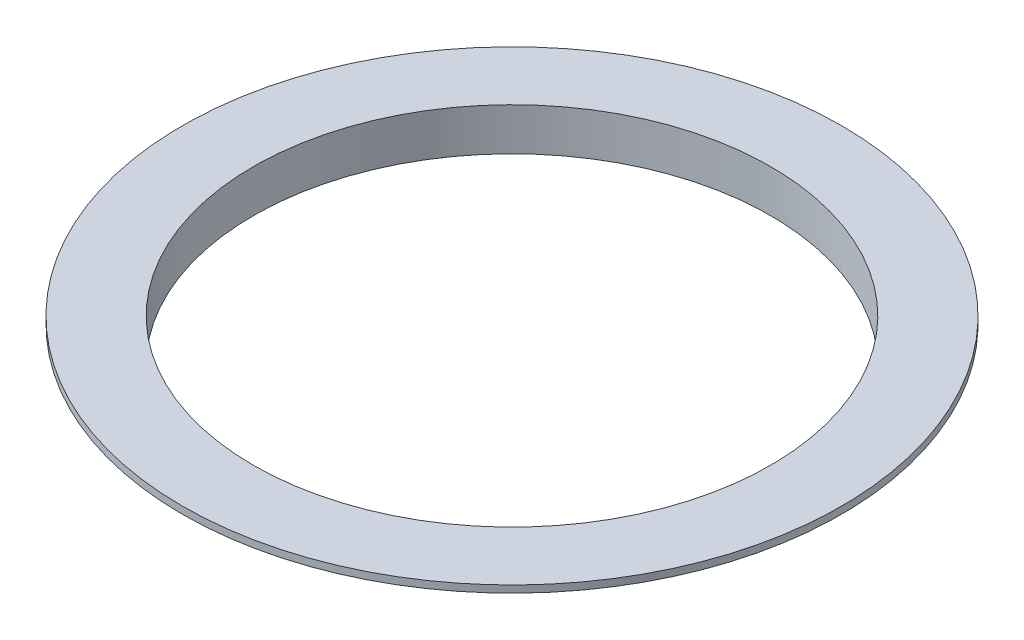
from build123d import *

# Parameters (mm, degrees)
SKETCH1_R           = 75
SKETCH1_R_2         = 73
BOSS_EXTRUDE1_DEPTH = 10
SKETCH3_R           = 93
SKETCH3_R_2         = 73
BOSS_EXTRUDE2_DEPTH = 2


with BuildPart() as part:
    # Sketch1 → Boss-Extrude1 (new body)
    with BuildSketch(Plane(origin=(0, 0, 0), x_dir=(1, 0, 0), z_dir=(0, 1, 0))):
        with Locations(Location((0, 0, 0), (0, 0, 270))):
            Circle(SKETCH1_R)
        with Locations(Location((0, 0, 0), (0, 0, 270))):
            Circle(SKETCH1_R_2, mode=Mode.SUBTRACT)
    extrude(amount=BOSS_EXTRUDE1_DEPTH)

    # Sketch3 → Boss-Extrude2 (add)
    with BuildSketch(Plane(origin=(0, 10, 0), x_dir=(1, 0, 0), z_dir=(0, 1, 0))):
        with Locations(Location((0, 0, 0), (0, 0, 270))):
            Circle(SKETCH3_R)
        with Locations(Location((0, 0, 0), (0, 0, 270))):
            Circle(SKETCH3_R_2, mode=Mode.SUBTRACT)
    extrude(amount=BOSS_EXTRUDE2_DEPTH)


solid = part.part
